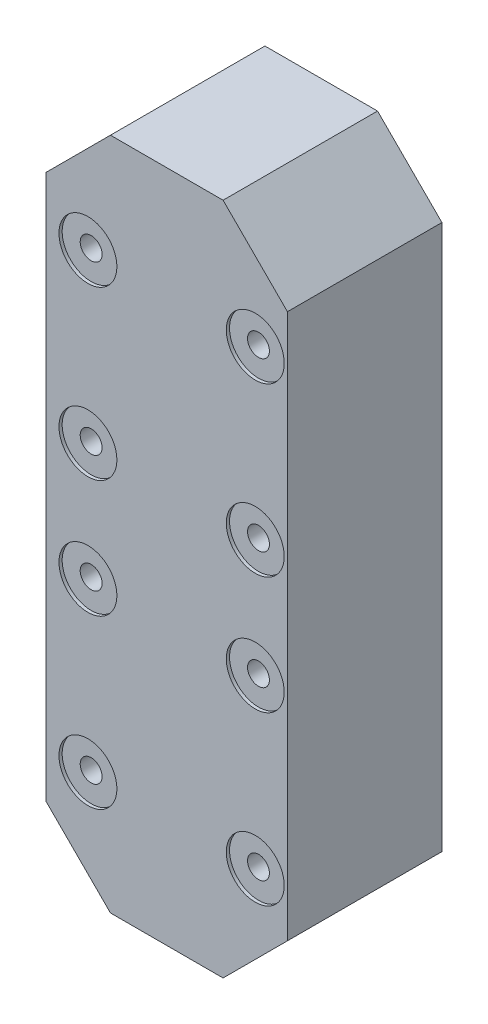
SolidWorks part; units mm, degrees
ref_plane "Front Plane" through (0, 0, 0) normal (0, 0, 1) x (1, 0, 0)
ref_plane "Top Plane" through (0, 0, 0) normal (0, 1, 0) x (1, 0, 0)
ref_plane "Right Plane" through (0, 0, 0) normal (1, 0, 0) x (0, 0, -1)
other "Configuration Table"
sketch "Sketch1" plane through (0, 0, 0) normal (0, 0, 1) x (1, 0, 0)
  line L0 (-17, 0) -> (-17, 39.4) construction
  line L1 (-19.5, 49.9) -> (18, 49.9)
  line L2 (-19.5, 49.9) -> (-19.5, -54.7571)
  line L3 (-19.5, -54.7571) -> (18, -54.7571)
  line L4 (18, 49.9) -> (18, -54.7571)
  line L5 (15.675, 48.9) -> (-15.675, 48.9) construction
  line L6 (17, 39.4) -> (17, 0) construction
  line L7 (-15.675, -53.7571) -> (15.675, -53.7571) construction
  dimension "D1" = 2.5
  dimension "D2" = 1
  dimension "D3" = 1
  dimension "D4" = 1
extrude "Boss-Extrude1" add sketch "Sketch1" along normal blind 24 and the other way blind 2
sketch "Sketch2" plane through (0, -54.7571, 0) normal (0, -1, 0) x (1, 0, 0)
  line L0 (-19.5, -2) -> (-19.5, 24) construction
  line L1 (18, -2) -> (-17, -2)
  line L2 (18, -2) -> (18, 0)
  line L3 (18, 0) -> (-17, 0)
  line L4 (-17, -2) -> (-17, 0)
  dimension "D1" = 2
  dimension "D2" = 2.5
extrude "Cut-Extrude1" cut sketch "Sketch2" against normal through all
chamfer "Chamfer1" distance 10 angle 45 4 edges at (18, -54.7571, 12) (-19.5, -54.7571, 11) (18, 49.9, 12) (-19.5, 49.9, 11)
sketch "Sketch3" plane through (0, 0, 24) normal (0, 0, 1) x (1, 0, 0)
hole_wizard "CBORE for M3 Hex Head Bolt1" positions "Sketch5" profile "Sketch4" counterbore size "M3" standard "GB" end condition through all
sketch "Sketch5" plane through (0, 0, 24) normal (0, 0, 1) x (1, 0, 0)
  point P0 (-13, 32.7)
  point P3 (13, 32.7)
  point P6 (13, 6.7)
  point P9 (-13, 6.7)
  point P12 (-13, -11.5571)
  point P15 (13, -11.5571)
  point P18 (13, -37.5571)
  point P21 (-13, -37.5571)
sketch "Sketch4" plane through (-13, 32.7, 24) normal (1, 0, 0) x (0, -1, 0)
  line L0 (0, 0) -> (0, 26)
  line L1 (0, 26) -> (1.7, 26)
  line L3 (1.7, 26) -> (1.7, 0.5)
  line L4 (1.7, 0.5) -> (4.5, 0.5)
  line L5 (4.5, 0.5) -> (4.5, 0)
  line L7 (4.5, 0) -> (0, 0)
  line L11 (0, -6.35) -> (0, 107.95) construction
  dimension "通孔孔直径" = 3.4
  dimension "通孔孔深度" = 26
  dimension "柱形沉头孔直径" = 9
  dimension "柱形沉头孔深度" = 0.5
